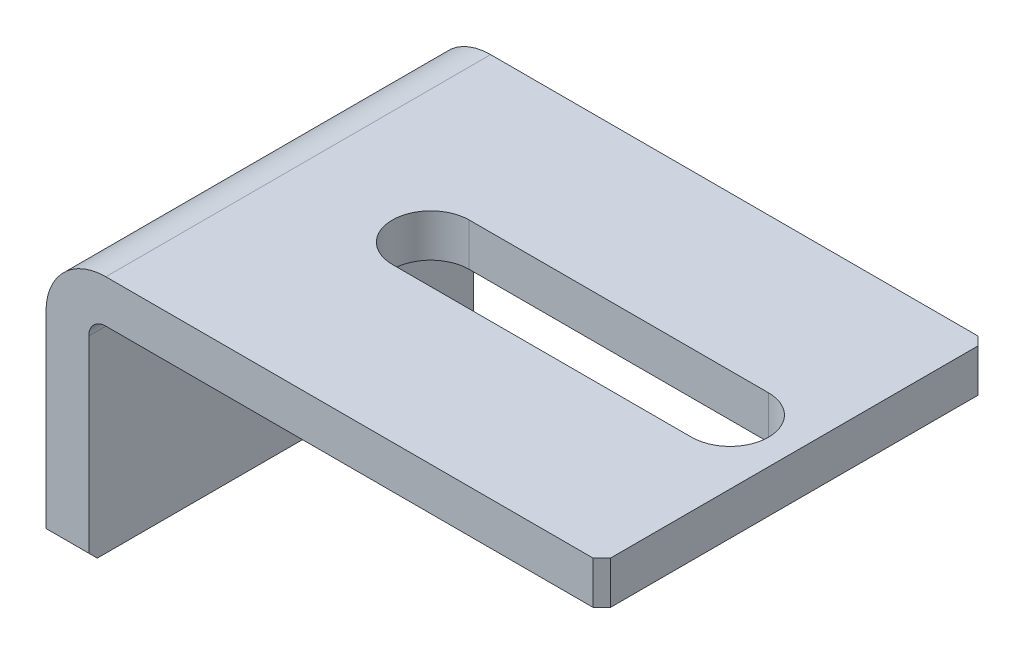
SolidWorks part; units mm, degrees
ref_plane "前视" through (0, 0, 0) normal (0, 0, 1) x (1, 0, 0)
ref_plane "上视" through (0, 0, 0) normal (0, 1, 0) x (1, 0, 0)
ref_plane "右视" through (0, 0, 0) normal (1, 0, 0) x (0, 0, -1)
sketch "草图1" plane through (0, 0, 0) normal (0, 0, 1) x (1, 0, 0)
  line L0 (0, 0) -> (0, 30)
  line L1 (0, 30) -> (65, 30)
  dimension "D1" = 30
  dimension "D2" = 65
extrude "拉伸-薄壁1" add sketch "草图1" along normal blind 45 thin
fillet "圆角1" radius 2 1 edges at (5, 25, 22.5)
fillet "圆角2" radius 7 1 edges at (0, 30, 22.5)
chamfer "倒角1" distance 1 angle 45 4 edges at (2.5, 0, 0) (2.5, 0, 45) (65, 27.5, 0) (65, 27.5, 45)
sketch "草图2" plane through (0, 30, 0) normal (0, 1, 0) x (1, 0, 0)
  line L0 (22.5, -22.5) -> (57.5, -22.5) construction
  line L1 (22.5, -18) -> (57.5, -18)
  line L2 (22.5, -27) -> (57.5, -27)
  line L3 (65, -22.5) -> (-20.5746, -22.5) construction
  line L4 (65, -44) -> (65, -1) construction
  arc A0 (22.5, -18) -> (22.5, -27) centre (22.5, -22.5) ccw
  arc A1 (57.5, -27) -> (57.5, -18) centre (57.5, -22.5) ccw
  point P2 (40, -22.5)
  dimension "D1" = 9
  dimension "D2" = 25
  dimension "D3" = 35
extrude "切除-拉伸1" cut sketch "草图2" against normal through all
